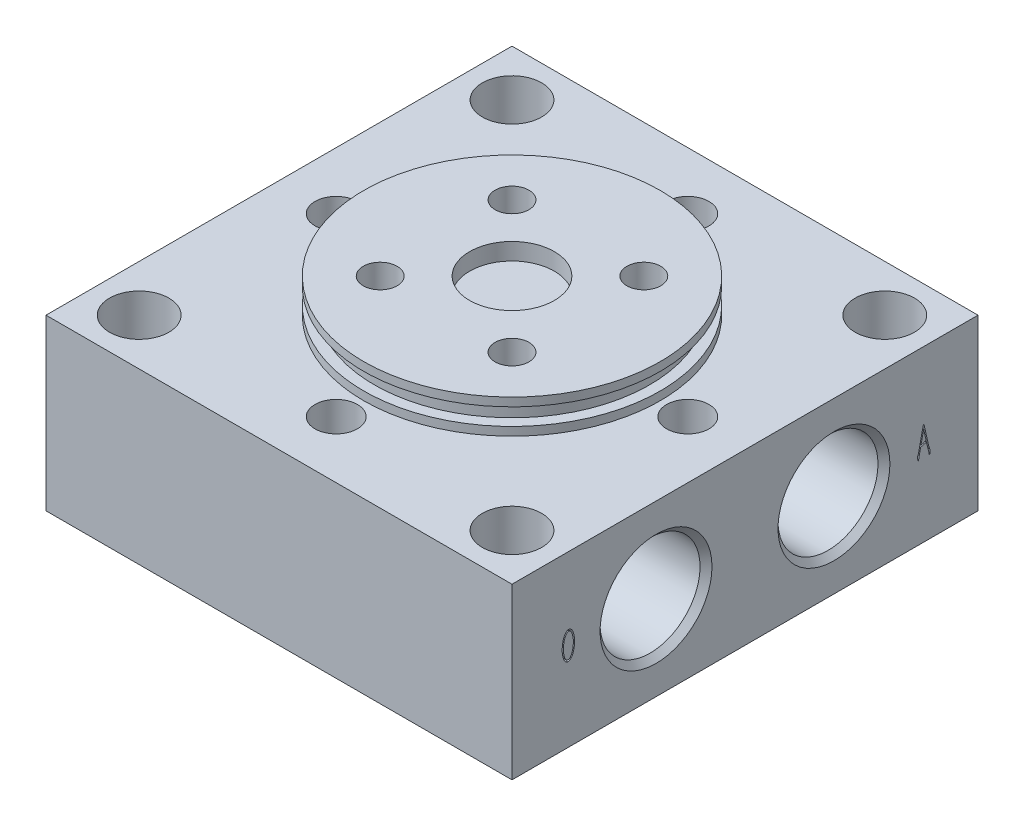
from build123d import *

# Parameters (mm, degrees)
SKETCH1_W               = 55
SKETCH1_H               = 55
BOSS_EXTRUDE1_DEPTH     = 10
SKETCH2_R               = 17.5
BOSS_EXTRUDE2_DEPTH     = 4
SKETCH3_R               = 5
CUT_EXTRUDE1_DEPTH      = 2
SKETCH4_W               = 1.25
SKETCH4_H               = 2
SKETCH9_R               = 3.5
CUT_EXTRUDE2_DEPTH      = 46.700109409
MIRROR4_COPY_1_SKETCH_R = 3.5
MIRROR4_COPY_1_DEPTH    = 46.700109409
CHAMFER1_SIZE           = 1
HOLE1_D                 = 5
HOLE1_DEPTH             = 100
HOLE1_CBORE_D           = 8.5
HOLE1_CBORE_DEPTH       = 3
CIRPATTERN1_COUNT       = 4
CHAMFER2_SIZE           = 1
CUT_EXTRUDE3_REACH      = 47.7
CUT_EXTRUDE3_END_RADIUS = 5.9
SKETCH12_R              = 2
CIRPATTERN2_COUNT       = 4
CUT_EXTRUDE4_DEPTH      = 1
CUT_EXTRUDE6_DEPTH      = 1
CUT_EXTRUDE7_DEPTH      = 1


with BuildPart() as part:
    # Sketch1 → Boss-Extrude1 (new, symmetric)
    with BuildSketch(Plane(origin=(0, 0, 0), x_dir=(1, 0, 0), z_dir=(0, 1, 0))):
        Rectangle(SKETCH1_W, SKETCH1_H)
    extrude(amount=BOSS_EXTRUDE1_DEPTH, both=True)

    # Sketch2 → Boss-Extrude2 (add)
    with BuildSketch(Plane(origin=(0, 10, 0), x_dir=(1, 0, 0), z_dir=(0, 1, 0))):
        with Locations(Location((0, 0, 0), (0, 0, 270))):
            Circle(SKETCH2_R)
    extrude(amount=BOSS_EXTRUDE2_DEPTH)

    # Sketch3 → Cut-Extrude1 (cut)
    with BuildSketch(Plane(origin=(0, 14, 0), x_dir=(1, 0, 0), z_dir=(0, 1, 0))):
        with Locations(Location((0, 0, 0), (0, 0, 270))):
            Circle(SKETCH3_R)
    extrude(amount=-CUT_EXTRUDE1_DEPTH, mode=Mode.SUBTRACT)

    # Sketch4 → Cut-Revolve1 (revolve, cut)
    with BuildSketch(Plane.XY, mode=Mode.PRIVATE) as cut_revolve1_sk:
        with Locations((-16.875, 12)):
            Rectangle(SKETCH4_W, SKETCH4_H)
    revolve(cut_revolve1_sk.sketch.rotate(Axis((0, 0, 0), (0, 1, 0)), 270), axis=Axis((0, 0, 0), (0, 1, 0)), mode=Mode.SUBTRACT)

    # Sketch6 → G1/4 Tapped Hole1 (revolve, cut)
    with BuildSketch(Plane(origin=(-27.5, 0, -10.5), x_dir=(0, 0, 1), z_dir=(0, 1, 0))):
        Polygon((0, 0), (0, 25.545077652), (5.9, 22), (5.9, 0.7035), (6.6035, 0), align=None)
    g1_4_tapped_hole1 = revolve(axis=Axis((-33.85, 0, -10.5), (1, 0, 0)), mode=Mode.SUBTRACT)

    # Mirror1: G1/4 Tapped Hole1 across plane
    add(g1_4_tapped_hole1.mirror(Plane.XY), mode=Mode.SUBTRACT)

    # Mirror2: G1/4 Tapped Hole1 across plane
    add(g1_4_tapped_hole1.mirror(Plane(origin=(0, 0, 0), x_dir=(0, 0, 1), z_dir=(1, 0, 0))), mode=Mode.SUBTRACT)

    # Mirror2 copy 1 sketch → Mirror2 copy 1 (revolve, cut)
    with BuildSketch(Plane(origin=(27.5, 0, 10.5), x_dir=(0, 0, -1), z_dir=(0, 1, 0))):
        Polygon((0, 0), (0, 25.545077652), (5.9, 22), (5.9, 0.7035), (6.6035, 0), align=None)
    revolve(axis=Axis((33.85, 0, 10.5), (-1, 0, 0)), mode=Mode.SUBTRACT)

    # Sketch9 → Cut-Extrude2 (cut, through all)
    with BuildSketch(Plane.XZ.offset(10)):
        with Locations(Location((22, 22, 0), (0, 0, 270))):
            Circle(SKETCH9_R)
    cut_extrude2 = extrude(amount=-CUT_EXTRUDE2_DEPTH, mode=Mode.SUBTRACT)

    # Mirror3: Cut-Extrude2 across plane
    add(cut_extrude2.mirror(Plane(origin=(0, 0, 0), x_dir=(0, 0, 1), z_dir=(1, 0, 0))), mode=Mode.SUBTRACT)

    # Mirror4: Cut-Extrude2 across plane
    add(cut_extrude2.mirror(Plane.XY), mode=Mode.SUBTRACT)

    # Mirror4 copy 1 sketch → Mirror4 copy 1 (cut, through all)
    with BuildSketch(Plane(origin=(0, -10, 0), x_dir=(-1, 0, 0), z_dir=(0, -1, 0))):
        with Locations(Location((22, 22, 0), (0, 0, 270))):
            Circle(MIRROR4_COPY_1_SKETCH_R)
    extrude(amount=-MIRROR4_COPY_1_DEPTH, mode=Mode.SUBTRACT)

    # Chamfer1
    chamfer1_edges = [part.edges().sort_by_distance(p)[0] for p in [
        (22, -10, 25.5),
        (-22, -10, 25.5),
        (-22, -10, -25.5),
        (22, -10, -25.5),
    ]]
    chamfer(chamfer1_edges, length=CHAMFER1_SIZE)

    # Hole1
    with Locations(Plane(origin=(0, -10, 0), x_dir=(-1, 0, 0), z_dir=(0, -1, 0))):
        with Locations((0, 20.75)):
            hole1 = CounterBoreHole(HOLE1_D / 2, HOLE1_CBORE_D / 2, HOLE1_CBORE_DEPTH, depth=HOLE1_DEPTH)

    # CirPattern1: Hole1 ×4 about axis
    cirpattern1_axis = Axis((0, 0, 0), (0, 1, 0))
    for i in range(1, CIRPATTERN1_COUNT):
        add(hole1.rotate(cirpattern1_axis, i * 360 / CIRPATTERN1_COUNT), mode=Mode.SUBTRACT)

    # Chamfer2
    chamfer2_edges = [part.edges().sort_by_distance(p)[0] for p in [
        (4.25, -10, -20.75),
        (20.75, -10, 4.25),
        (-4.25, -10, 20.75),
        (-20.75, -10, -4.25),
    ]]
    chamfer(chamfer2_edges, length=CHAMFER2_SIZE)

    # Cut-Extrude3: up to this cylinder (the profile starts outside it)
    cut_extrude3_end = Plane(origin=(-7.778175, 0, -10.5), z_dir=(-1, 0, 0)) * Cylinder(CUT_EXTRUDE3_END_RADIUS, 108.2, mode=Mode.PRIVATE)
    # Sketch12 → Cut-Extrude3 (cut, up to the surface)
    with BuildSketch(Plane(origin=(0, 14, 0), x_dir=(1, 0, 0), z_dir=(0, 1, 0)), mode=Mode.PRIVATE) as cut_extrude3_sk1:
        with Locations(Location((-7.778174593, 7.778174593, 0), (0, 0, 270))):
            Circle(SKETCH12_R)
    cut_extrude3_tool1 = extrude(cut_extrude3_sk1.sketch, amount=-CUT_EXTRUDE3_REACH, mode=Mode.PRIVATE) - cut_extrude3_end
    cut_extrude3 = cut_extrude3_tool1.solids().sort_by_distance((-7.778175, 14, -7.778175))[0]
    add(cut_extrude3, mode=Mode.SUBTRACT)

    # CirPattern2: Cut-Extrude3 ×4 about axis
    cirpattern2_axis = Axis((0, 0, 0), (0, 1, 0))
    for i in range(1, CIRPATTERN2_COUNT):
        add(cut_extrude3.rotate(cirpattern2_axis, i * 360 / CIRPATTERN2_COUNT), mode=Mode.SUBTRACT)

    # Sketch13 → Cut-Extrude4 (cut)
    with BuildSketch(Plane(origin=(27.5, 0, 0), x_dir=(0, 0, -1), z_dir=(1, 0, 0))):
        with BuildLine():
            Line((21.41827741, 0.056894821), (20.733640717, -0.108670916))
            Line((20.733640717, -0.108670916), (20.572549731, -0.85893727))
            Line((20.572549731, -0.85893727), (20.496478987, -1.241528363))
            Line((20.496478987, -1.241528363), (20.466647323, -1.362346603))
            add(Edge.make_bspline(
                [(20.466647323, -1.362346603), (20.463479594, -1.370904686), (20.458137517, -1.385337094), (20.448085785, -1.402316971), (20.437055284, -1.410755091), (20.424739604, -1.412533881), (20.415500199, -1.401854686), (20.410006027, -1.388320722), (20.408361513, -1.368459439), (20.40379183, -1.342600787), (20.400934079, -1.305609162), (20.397654946, -1.277557618), (20.395797121, -1.261664736)],
                knots=[0, 0, 0, 0, 1.226577759, 2.068508672, 2.595953142, 3.064162245, 3.560072257, 4.322224954, 5.029865969, 6.20926766, 7.852322798, 10, 10, 10, 10], degree=3))
            Line((20.395797121, -1.261664736), (20.371185998, -1.050605712))
            add(Edge.make_bspline(
                [(20.371185998, -1.050605712), (20.369595159, -1.033213536), (20.366757091, -1.002185763), (20.364263432, -0.961134647), (20.364101522, -0.931516715), (20.365536736, -0.906738529), (20.37287408, -0.883306403), (20.381590798, -0.867247825), (20.38610183, -0.85893727)],
                knots=[0, 0, 0, 0, 1.603576797, 2.86079302, 3.773774944, 4.323462854, 5.1323669, 6, 6, 6, 6], degree=3))
            Line((20.38610183, -0.85893727), (20.411458744, -0.813443982))
            add(Edge.make_bspline(
                [(20.411458744, -0.813443982), (20.416889513, -0.801595135), (20.429859356, -0.773297545), (20.446281631, -0.721203273), (20.463777805, -0.653375719), (20.481407717, -0.575307408), (20.498689018, -0.499704987), (20.512494693, -0.438103226), (20.523090834, -0.397241397), (20.529982216, -0.377138015), (20.532276984, -0.370443769)],
                knots=[0, 0, 0, 0, 0.679694972, 1.623257572, 2.844174753, 4.335796169, 5.799225578, 6.891200865, 7.630779852, 8, 8, 8, 8], degree=3))
            Line((20.532276984, -0.370443769), (21.050602149, 2.030259406))
            Line((21.050602149, 2.030259406), (21.12070656, 2.030259406))
            Line((21.12070656, 2.030259406), (21.609200061, -0.128807289))
            Line((21.609200061, -0.128807289), (21.669609181, -0.380884851))
            add(Edge.make_bspline(
                [(21.669609181, -0.380884851), (21.675668779, -0.4092612), (21.68653881, -0.460164213), (21.703079907, -0.52776564), (21.716645868, -0.578389221), (21.726184983, -0.606146467), (21.730018301, -0.61730079)],
                knots=[0, 0, 0, 0, 1.425899692, 2.557855139, 3.420470246, 4, 4, 4, 4], degree=3))
            Line((21.730018301, -0.61730079), (21.765070506, -0.712762115))
            add(Edge.make_bspline(
                [(21.765070506, -0.712762115), (21.769105272, -0.726745828), (21.77645646, -0.752223612), (21.789013801, -0.785943136), (21.80135485, -0.811979223), (21.817068063, -0.833907011), (21.833006758, -0.850364641), (21.844008493, -0.867431963), (21.845398376, -0.883364804), (21.84347131, -0.897971275), (21.841413369, -0.916574349), (21.840412026, -0.939998551), (21.837753743, -0.972271763), (21.836579468, -0.996654459), (21.835920709, -1.010332965)],
                knots=[0, 0, 0, 0, 1.645080438, 2.997272953, 4.065812928, 4.892545225, 6.029861332, 6.67147811, 7.124734071, 7.80170629, 8.338742145, 9.240009017, 10.451666043, 12, 12, 12, 12], degree=3))
            Line((21.835920709, -1.010332965), (21.815784336, -1.236307822))
            Line((21.815784336, -1.236307822), (21.805343253, -1.322073856))
            add(Edge.make_bspline(
                [(21.805343253, -1.322073856), (21.804846829, -1.331800262), (21.803964414, -1.349089378), (21.799710387, -1.371359831), (21.796925261, -1.387525447), (21.791057653, -1.399220748), (21.779909712, -1.405003708), (21.766089397, -1.400970109), (21.755467273, -1.386991211), (21.752111389, -1.374721336), (21.750154674, -1.367567144)],
                knots=[0, 0, 0, 0, 1.663187075, 2.956388731, 3.874273883, 4.464983498, 5.130530035, 5.83179128, 6.735783313, 8, 8, 8, 8], degree=3))
            Line((21.750154674, -1.367567144), (21.715102469, -1.166203411))
            Line((21.715102469, -1.166203411), (21.41827741, 0.056894821))
        make_face()
        with BuildLine():
            Line((21.407836328, 0.132965564), (21.085654355, 1.546986446))
            Line((21.085654355, 1.546986446), (20.75825184, 0.067335903))
            add(Edge.make_bspline(
                [(20.75825184, 0.067335903), (20.786653818, 0.071713699), (20.835687119, 0.079271544), (20.904028724, 0.094281317), (20.968709563, 0.112048218), (21.026146573, 0.127940621), (21.073590406, 0.14406318), (21.104589464, 0.154731291), (21.128139648, 0.165754404), (21.140665789, 0.174111761), (21.146063475, 0.177713061)],
                knots=[0, 0, 0, 0, 1.70172219, 2.937860729, 4.141475294, 5.674569601, 6.46612829, 7.108957565, 7.616037637, 8, 8, 8, 8], degree=3))
            Line((21.146063475, 0.177713061), (21.272102256, 0.263479095))
            Line((21.272102256, 0.263479095), (21.407836328, 0.132965564))
        make_face(mode=Mode.SUBTRACT)
    extrude(amount=-CUT_EXTRUDE4_DEPTH, mode=Mode.SUBTRACT)

    # Sketch14 → Cut-Extrude6 (cut)
    with BuildSketch(Plane(origin=(27.5, 0, 0), x_dir=(0, 0, -1), z_dir=(1, 0, 0))):
        with BuildLine():
            add(Edge.make_bspline(
                [(-21.573757582, 0.463669295), (-21.570691446, 0.511932871), (-21.564373449, 0.611383491), (-21.546495118, 0.764033475), (-21.523391202, 0.924733609), (-21.494531327, 1.089931426), (-21.45842848, 1.253615372), (-21.409140298, 1.406968714), (-21.350380038, 1.548232182), (-21.280957443, 1.673587805), (-21.208198436, 1.781766032), (-21.137917897, 1.870157478), (-21.071763548, 1.938118373), (-21.006582548, 1.983823464), (-20.944517431, 2.012043895), (-20.887579323, 2.031645432), (-20.834254477, 2.044425119), (-20.799687025, 2.044138334), (-20.783218481, 2.044001705)],
                knots=[0, 0, 0, 0, 1.217793816, 2.509352989, 3.869389901, 5.306369188, 6.732518591, 8.086865491, 9.357865112, 10.57959578, 11.689225504, 12.637700741, 13.421327601, 14.069152645, 14.629329011, 15.132240194, 15.586583926, 16, 16, 16, 16], degree=3))
            add(Edge.make_bspline(
                [(-20.783218481, 2.044001705), (-20.767426973, 2.041261552), (-20.733849942, 2.035435245), (-20.682789884, 2.015383688), (-20.627615703, 1.987897956), (-20.569705453, 1.950672135), (-20.51151679, 1.90327457), (-20.456490892, 1.843520338), (-20.406791008, 1.771014125), (-20.345589446, 1.658264953), (-20.278997371, 1.503374055), (-20.226466165, 1.338747987), (-20.19239833, 1.199951602), (-20.16889652, 1.089116308), (-20.149948201, 0.972064152), (-20.128312505, 0.80900423), (-20.108857675, 0.601811935), (-20.111955861, 0.435372211), (-20.11349762, 0.352546346)],
                knots=[0, 0, 0, 0, 0.394985608, 0.839846589, 1.347857167, 1.916750551, 2.536277094, 3.196746505, 3.915575437, 4.701623328, 6.36253532, 8.071356979, 8.963406565, 9.891884595, 10.869033514, 11.891140732, 13.955296867, 16, 16, 16, 16], degree=3))
            add(Edge.make_bspline(
                [(-20.11349762, 0.352546346), (-20.114789645, 0.321461233), (-20.117469781, 0.256979241), (-20.125601646, 0.157428876), (-20.139029229, 0.051884429), (-20.159125682, -0.097503151), (-20.196773191, -0.288653981), (-20.248813642, -0.478020533), (-20.299959181, -0.626162428), (-20.343875525, -0.731714709), (-20.392424734, -0.831888465), (-20.446108546, -0.924275466), (-20.50188653, -1.007422099), (-20.561638755, -1.076348685), (-20.622032408, -1.131723757), (-20.684965724, -1.17077827), (-20.74573499, -1.197352301), (-20.802093274, -1.215837832), (-20.854774052, -1.224903531), (-20.888103078, -1.223826305), (-20.904036721, -1.223311315)],
                knots=[0, 0, 0, 0, 0.881282943, 1.828105941, 2.82824081, 3.894865892, 6.097710261, 8.340987808, 9.452332789, 10.535200188, 11.577677107, 12.603151353, 13.560288859, 14.408919748, 15.182050945, 15.871786862, 16.496001568, 17.057257397, 17.549302039, 18, 18, 18, 18], degree=3))
            add(Edge.make_bspline(
                [(-20.904036721, -1.223311315), (-20.920550298, -1.221349209), (-20.955215733, -1.217230342), (-21.008123304, -1.199662765), (-21.064025867, -1.173173265), (-21.123094658, -1.137571684), (-21.182895081, -1.089677604), (-21.238402903, -1.02552304), (-21.292412395, -0.948198037), (-21.341946304, -0.856675456), (-21.388278542, -0.754904909), (-21.429707213, -0.64507945), (-21.467077085, -0.529109163), (-21.499540849, -0.408405105), (-21.525554664, -0.285756755), (-21.547809745, -0.16551661), (-21.562311551, -0.048680046), (-21.572466566, 0.063757537), (-21.576060976, 0.171547051), (-21.578741939, 0.273970972), (-21.578200055, 0.370740853), (-21.575207138, 0.43334721), (-21.573757582, 0.463669295)],
                knots=[0, 0, 0, 0, 0.510534934, 1.071719088, 1.704710998, 2.411693894, 3.189282936, 4.05053371, 5.011670478, 6.086573801, 7.246791516, 8.449877322, 9.695482973, 10.994127406, 12.29322218, 13.551907867, 14.754774865, 15.913908135, 17.0238299, 18.071869134, 19.066149983, 20, 20, 20, 20], degree=3))
        make_face()
        with BuildLine():
            add(Edge.make_bspline(
                [(-21.427582427, 0.453228212), (-21.428993902, 0.42837503), (-21.431970413, 0.375964764), (-21.433120165, 0.293132799), (-21.432450524, 0.202116471), (-21.427658159, 0.068578079), (-21.41028584, -0.107700957), (-21.379671203, -0.28600609), (-21.345210741, -0.427946487), (-21.315480687, -0.529686707), (-21.282797293, -0.626028097), (-21.246040906, -0.714982753), (-21.206989611, -0.795194849), (-21.16389052, -0.86269606), (-21.120795203, -0.919498218), (-21.07284554, -0.96095983), (-21.026449208, -0.993065397), (-20.981582585, -1.014859935), (-20.939913724, -1.031579991), (-20.912122244, -1.035152811), (-20.89881618, -1.036863414)],
                knots=[0, 0, 0, 0, 0.796536737, 1.679732718, 2.650327695, 3.709147218, 5.954918549, 8.313069364, 9.492003862, 10.627402775, 11.704181224, 12.745734999, 13.706334556, 14.553839847, 15.30675304, 15.97732542, 16.573080319, 17.10674674, 17.572326302, 18, 18, 18, 18], degree=3))
            add(Edge.make_bspline(
                [(-20.89881618, -1.036863414), (-20.885116088, -1.03766974), (-20.856757889, -1.039338778), (-20.813193016, -1.030783983), (-20.767605376, -1.015733546), (-20.720395542, -0.991454463), (-20.671471858, -0.956768819), (-20.624678335, -0.906675445), (-20.577997255, -0.843572885), (-20.532200589, -0.768401348), (-20.48815732, -0.685034131), (-20.449030213, -0.595717941), (-20.412653191, -0.503480042), (-20.372741813, -0.374175287), (-20.328733755, -0.207848896), (-20.294142862, -0.00469703), (-20.270054835, 0.193469365), (-20.257219824, 0.354343807), (-20.255310839, 0.482324845), (-20.257833517, 0.585540018), (-20.263512534, 0.697752569), (-20.2708083, 0.775432835), (-20.274588607, 0.815682932)],
                knots=[0, 0, 0, 0, 0.389303871, 0.805830913, 1.253424913, 1.753499798, 2.311288848, 2.951911425, 3.695005091, 4.54345845, 5.455166886, 6.377091015, 7.318103512, 8.276048787, 10.227707478, 12.21152619, 14.136557685, 15.91040834, 16.802233067, 17.779101204, 18.849239395, 20, 20, 20, 20], degree=3))
            add(Edge.make_bspline(
                [(-20.274588607, 0.815682932), (-20.278749151, 0.85227031), (-20.286835512, 0.923380897), (-20.303712465, 1.025706179), (-20.321026259, 1.121196747), (-20.349319536, 1.238195031), (-20.390241956, 1.379672869), (-20.442858772, 1.515193259), (-20.490824524, 1.617126524), (-20.529489874, 1.683357874), (-20.573518157, 1.737161993), (-20.619504542, 1.779802429), (-20.666198859, 1.811647703), (-20.71008361, 1.836185545), (-20.752407674, 1.852061459), (-20.780378775, 1.855785577), (-20.793659563, 1.857553804)],
                knots=[0, 0, 0, 0, 1.251575308, 2.432539829, 3.524812851, 4.549720602, 6.523204923, 8.527303315, 9.483611249, 10.351763581, 11.126540771, 11.838283349, 12.475927762, 13.043152764, 13.545685196, 14, 14, 14, 14], degree=3))
            add(Edge.make_bspline(
                [(-20.793659563, 1.857553804), (-20.8066188, 1.85661231), (-20.834081233, 1.854617153), (-20.876887901, 1.845024545), (-20.921372027, 1.825740368), (-20.971141922, 1.802471809), (-21.023638907, 1.76325926), (-21.076807726, 1.704111951), (-21.132758519, 1.62563128), (-21.192555488, 1.530306852), (-21.249824351, 1.418473241), (-21.296642695, 1.290920724), (-21.33756029, 1.151604218), (-21.365700214, 1.002386979), (-21.389120424, 0.853049539), (-21.406566885, 0.710439818), (-21.421041536, 0.578506064), (-21.425465251, 0.49377853), (-21.427582427, 0.453228212)],
                knots=[0, 0, 0, 0, 0.37757334, 0.800130614, 1.267198275, 1.784369715, 2.394414205, 3.156344445, 4.08734282, 5.194407036, 6.425938495, 7.73207238, 9.1388751, 10.642807986, 12.142427514, 13.533772035, 14.819671431, 16, 16, 16, 16], degree=3))
        make_face(mode=Mode.SUBTRACT)
    extrude(amount=-CUT_EXTRUDE6_DEPTH, mode=Mode.SUBTRACT)

    # Sketch15 → Cut-Extrude7 (cut)
    # profile 1 of 2: a face of its own
    with BuildSketch(Plane.ZY.offset(27.5)):
        with BuildLine():
            add(Edge.make_bspline(
                [(-22.716854148, 1.943319838), (-22.678283366, 1.949836343), (-22.604277282, 1.962339617), (-22.496871122, 1.983743416), (-22.393200184, 2.001804845), (-22.324140124, 2.006563605), (-22.289515559, 2.008949499)],
                knots=[0, 0, 0, 0, 1.084781132, 2.081378719, 3.038062992, 4, 4, 4, 4], degree=3))
            add(Edge.make_bspline(
                [(-22.289515559, 2.008949499), (-22.269612591, 2.009379341), (-22.231712494, 2.010197864), (-22.178043644, 2.004711516), (-22.130099478, 1.99577851), (-22.087718008, 1.979371435), (-22.048808231, 1.957200452), (-22.011532761, 1.927956184), (-21.975273294, 1.891371922), (-21.939913694, 1.846869118), (-21.906856359, 1.79404757), (-21.879514156, 1.73085753), (-21.856212079, 1.658519117), (-21.835491489, 1.550364095), (-21.815180708, 1.414048318), (-21.808170117, 1.279654783), (-21.80790067, 1.179100032), (-21.810863807, 1.11041887), (-21.816441375, 1.046873921), (-21.823154397, 1.006573268), (-21.826378972, 0.987215001)],
                knots=[0, 0, 0, 0, 0.834042403, 1.588219797, 2.258865872, 2.872645434, 3.484296274, 4.130763207, 4.85321558, 5.639635085, 6.510463327, 7.457868132, 8.519533185, 9.691141985, 12.070813463, 14.294972691, 15.327100164, 16.287155067, 17.177241371, 18, 18, 18, 18], degree=3))
            add(Edge.make_bspline(
                [(-21.826378972, 0.987215001), (-21.830486178, 0.964508438), (-21.83849221, 0.92024733), (-21.856297246, 0.85702977), (-21.875017714, 0.797567908), (-21.89836069, 0.74383886), (-21.922884912, 0.694379821), (-21.950358068, 0.650866263), (-21.97950663, 0.611880349), (-22.0214278, 0.569497691), (-22.077733739, 0.526608018), (-22.151540319, 0.493581811), (-22.226174894, 0.477633394), (-22.275286261, 0.474762931), (-22.299210849, 0.473364586)],
                knots=[0, 0, 0, 0, 1.080384674, 2.105956013, 3.074594822, 3.998289199, 4.84730105, 5.658400013, 6.406150959, 7.122683501, 8.445750941, 9.696890862, 10.878041055, 12, 12, 12, 12], degree=3))
            Line((-22.299210849, 0.473364586), (-22.495354041, 0.463669295))
            Line((-22.495354041, 0.463669295), (-22.757126895, 0.427871298))
            Line((-22.757126895, 0.427871298), (-22.762347436, -0.921265715))
            add(Edge.make_bspline(
                [(-22.762347436, -0.921265715), (-22.762913705, -0.951104576), (-22.76393324, -1.004827776), (-22.767620667, -1.076370903), (-22.768976187, -1.130408058), (-22.773464208, -1.180316008), (-22.778647003, -1.235510532), (-22.785967882, -1.288051036), (-22.791634518, -1.329651282), (-22.797623402, -1.34918199), (-22.802940506, -1.365782803), (-22.810361882, -1.364670505), (-22.813061265, -1.364265928)],
                knots=[0, 0, 0, 0, 1.96874048, 3.54460707, 4.726507013, 5.532831549, 6.851459339, 8.37313705, 9.071482733, 9.549088405, 9.835989539, 10, 10, 10, 10], degree=3))
            add(Edge.make_bspline(
                [(-22.813061265, -1.364265928), (-22.814050257, -1.363515116), (-22.818283382, -1.360301457), (-22.828625097, -1.353594461), (-22.839143721, -1.334273174), (-22.844737765, -1.318094511), (-22.84811347, -1.308331558)],
                knots=[0, 0, 0, 0, 0.220639879, 0.944392497, 2.156105254, 4, 4, 4, 4], degree=3))
            Line((-22.84811347, -1.308331558), (-22.873470385, -1.243447688))
            Line((-22.873470385, -1.243447688), (-22.933879505, -1.062220328))
            add(Edge.make_bspline(
                [(-22.933879505, -1.062220328), (-22.939513362, -1.044804713), (-22.94933033, -1.014458094), (-22.962969508, -0.975502701), (-22.969638556, -0.949202442), (-22.973423325, -0.928583645), (-22.964353832, -0.908163009), (-22.952948275, -0.880410812), (-22.937203358, -0.844065308), (-22.925904097, -0.799188809), (-22.915119575, -0.751163059), (-22.905346196, -0.700553929), (-22.899308598, -0.644979539), (-22.897724549, -0.591886551), (-22.898520003, -0.539408434), (-22.895984535, -0.48698194), (-22.896276463, -0.423306829), (-22.894540329, -0.377082761), (-22.893606758, -0.352226721)],
                knots=[0, 0, 0, 0, 1.21093634, 2.110050319, 2.719907809, 3.017552618, 3.464624392, 4.142243825, 5.027278712, 6.067997939, 7.196380019, 8.282686609, 9.473265847, 10.887508473, 11.791416163, 12.942313598, 14.355792079, 16, 16, 16, 16], degree=3))
            Line((-22.893606758, -0.352226721), (-22.883165676, 1.721819732))
            add(Edge.make_bspline(
                [(-22.883165676, 1.721819732), (-22.89393359, 1.743438266), (-22.913721033, 1.783165134), (-22.946094396, 1.833417418), (-22.971246853, 1.87169286), (-22.984027246, 1.9020465), (-22.987699799, 1.92482587), (-22.988644728, 1.937597694), (-22.989068084, 1.943319838)],
                knots=[0, 0, 0, 0, 1.750659444, 3.217064329, 4.333728491, 5.070582308, 5.583594197, 6, 6, 6, 6], degree=3))
            add(Edge.make_bspline(
                [(-22.989068084, 1.943319838), (-22.988395861, 1.946273967), (-22.986846978, 1.953080635), (-22.974941937, 1.958979274), (-22.95853723, 1.959110016), (-22.94582175, 1.958559169), (-22.938354254, 1.95823567)],
                knots=[0, 0, 0, 0, 0.599620471, 1.381597738, 2.462275397, 4, 4, 4, 4], degree=3))
            Line((-22.938354254, 1.95823567), (-22.888386217, 1.948540379))
            Line((-22.888386217, 1.948540379), (-22.716854148, 1.943319838))
        make_face()
        with BuildLine():
            Line((-22.757126895, 0.604623908), (-22.420029089, 0.639676113))
            add(Edge.make_bspline(
                [(-22.420029089, 0.639676113), (-22.389659167, 0.64277566), (-22.325531551, 0.649320508), (-22.24450315, 0.664153492), (-22.17912965, 0.68387545), (-22.132739522, 0.703769588), (-22.092221091, 0.730318638), (-22.056122995, 0.761985542), (-22.026096533, 0.801171941), (-22.000039453, 0.846962008), (-21.98233073, 0.901671976), (-21.963625288, 0.984329257), (-21.950018717, 1.095916352), (-21.948147345, 1.187053907), (-21.947197212, 1.233326231)],
                knots=[0, 0, 0, 0, 1.242290402, 2.623158502, 3.343124827, 4.017967388, 4.668958523, 5.306607609, 5.962297971, 6.668776287, 7.439809609, 8.291324773, 10.117032856, 12, 12, 12, 12], degree=3))
            add(Edge.make_bspline(
                [(-21.947197212, 1.233326231), (-21.949190047, 1.262682698), (-21.953081569, 1.320008764), (-21.962820803, 1.403109396), (-21.975159968, 1.481396301), (-21.991809279, 1.553409649), (-22.008933129, 1.618648883), (-22.031858427, 1.673582275), (-22.055811912, 1.719079423), (-22.084068796, 1.755260629), (-22.117983756, 1.781769735), (-22.155541079, 1.804450295), (-22.200583979, 1.818616365), (-22.232522474, 1.824593178), (-22.249242812, 1.827722139)],
                knots=[0, 0, 0, 0, 1.450841259, 2.833141438, 4.12506739, 5.356415584, 6.477956507, 7.445537896, 8.28503356, 9.008768821, 9.688489171, 10.397114349, 11.160862483, 12, 12, 12, 12], degree=3))
            add(Edge.make_bspline(
                [(-22.249242812, 1.827722139), (-22.271617187, 1.828905835), (-22.317132287, 1.83131377), (-22.387413565, 1.826636657), (-22.460791645, 1.818330974), (-22.510339715, 1.807760111), (-22.535626788, 1.802365225)],
                knots=[0, 0, 0, 0, 0.931107193, 1.894105981, 2.925247858, 4, 4, 4, 4], degree=3))
            Line((-22.535626788, 1.802365225), (-22.742211062, 1.756871937))
            Line((-22.742211062, 1.756871937), (-22.757126895, 0.604623908))
        make_face(mode=Mode.SUBTRACT)
    # profile 2 of 2: a face of its own
    with BuildSketch(Plane.ZY.offset(27.5)):
        with BuildLine():
            add(Edge.make_bspline(
                [(21.693628067, 1.691988067), (21.68144982, 1.701426351), (21.659363699, 1.718543354), (21.626261092, 1.744287943), (21.595203373, 1.778112565), (21.566001926, 1.809561073), (21.542963494, 1.838354352), (21.531298815, 1.857622523), (21.523402988, 1.872579283), (21.5246256, 1.887945488), (21.533040377, 1.899696569), (21.541193258, 1.915088033), (21.563602484, 1.919215799), (21.588357215, 1.909906461), (21.614687366, 1.902080584), (21.635412693, 1.895266882), (21.653617141, 1.894705762), (21.675240608, 1.894612962), (21.706296294, 1.896767623), (21.744122071, 1.89751905), (21.782487322, 1.900134297), (21.815655143, 1.904454798), (21.841014373, 1.906760924), (21.85451463, 1.91155979), (21.859939594, 1.913488174)],
                knots=[0, 0, 0, 0, 1.64763205, 2.988098512, 4.472525849, 6.542356651, 7.584071831, 8.395257026, 8.967619365, 9.340564694, 9.97047718, 10.50190227, 11.107820098, 12.171334353, 13.314207223, 14.055349962, 14.481319576, 15.251885957, 16.369143228, 17.804974755, 19.296756072, 20.473415709, 21.386554954, 22, 22, 22, 22], degree=3))
            Line((21.859939594, 1.913488174), (22.112017157, 1.978372043))
            add(Edge.make_bspline(
                [(22.112017157, 1.978372043), (22.119702955, 1.98044976), (22.136711154, 1.98504762), (22.165526756, 1.990525658), (22.199458045, 1.998322566), (22.237580097, 2.005832569), (22.275388858, 2.014366522), (22.309884837, 2.018912641), (22.338365704, 2.023636951), (22.355627879, 2.02379475), (22.363348927, 2.023865331)],
                knots=[0, 0, 0, 0, 0.746644526, 1.652278328, 2.750112717, 4.012480095, 5.297690843, 6.382818677, 7.276664985, 8, 8, 8, 8], degree=3))
            add(Edge.make_bspline(
                [(22.363348927, 2.023865331), (22.37982691, 2.022072977), (22.412751277, 2.018491706), (22.461110029, 2.005058118), (22.507028119, 1.982656487), (22.550925834, 1.953858233), (22.59095464, 1.917821047), (22.627459229, 1.876311777), (22.658758162, 1.828330499), (22.684805886, 1.773689163), (22.706945512, 1.71319037), (22.72584969, 1.645908965), (22.740102535, 1.571731472), (22.751667489, 1.492807566), (22.760330626, 1.413671477), (22.766178377, 1.338293148), (22.770179572, 1.268917079), (22.770935959, 1.224630002), (22.771296935, 1.203494566)],
                knots=[0, 0, 0, 0, 0.788100513, 1.574689806, 2.373814472, 3.210589555, 4.065404581, 4.929098289, 5.834801075, 6.781980012, 7.803943584, 8.897694274, 10.10426717, 11.396006919, 12.693423483, 13.892139677, 14.994050896, 16, 16, 16, 16], degree=3))
            add(Edge.make_bspline(
                [(22.771296935, 1.203494566), (22.769145225, 1.169656343), (22.764799581, 1.10131587), (22.751972016, 0.997937392), (22.732724057, 0.891869128), (22.709802435, 0.804084814), (22.688794175, 0.738272076), (22.672903369, 0.698999764), (22.658719328, 0.668878774), (22.645550138, 0.65512756), (22.640037613, 0.649371404)],
                knots=[0, 0, 0, 0, 1.41233288, 2.852380741, 4.337314802, 5.89979107, 6.630150315, 7.21096505, 7.669715816, 8, 8, 8, 8], degree=3))
            Line((22.640037613, 0.649371404), (22.534880996, 0.544214788))
            add(Edge.make_bspline(
                [(22.534880996, 0.544214788), (22.557565411, 0.528722792), (22.598608356, 0.500693102), (22.645071678, 0.461390329), (22.678319315, 0.427877598), (22.70281792, 0.394674541), (22.73083987, 0.354139497), (22.770492123, 0.288189414), (22.817818257, 0.194199685), (22.847914883, 0.088254297), (22.866218398, -0.004931345), (22.873392474, -0.084855293), (22.878294161, -0.17292535), (22.877574807, -0.234383111), (22.877199343, -0.266460686)],
                knots=[0, 0, 0, 0, 1.070182896, 1.936283469, 2.368030692, 2.906882123, 3.541225939, 4.289096852, 5.905680189, 7.625612947, 8.562596306, 9.604952081, 10.749916543, 12, 12, 12, 12], degree=3))
            add(Edge.make_bspline(
                [(22.877199343, -0.266460686), (22.8759769, -0.296803371), (22.873598293, -0.355843629), (22.865639768, -0.442058005), (22.852471261, -0.523298732), (22.837622633, -0.60003388), (22.817272823, -0.671322376), (22.793079988, -0.736902963), (22.763747766, -0.796750681), (22.729229762, -0.850591225), (22.690355116, -0.89946799), (22.646336534, -0.943206688), (22.597905074, -0.982730633), (22.544625307, -1.017813007), (22.487612402, -1.048444602), (22.426168859, -1.072985294), (22.361430264, -1.093488422), (22.316221662, -1.102425553), (22.293244517, -1.106967824)],
                knots=[0, 0, 0, 0, 1.291181941, 2.512358873, 3.678492505, 4.789671877, 5.833657235, 6.827132701, 7.758433233, 8.661592748, 9.541502867, 10.408556622, 11.295108621, 12.19516981, 13.117306623, 14.041863747, 15.004782726, 16, 16, 16, 16], degree=3))
            Line((22.293244517, -1.106967824), (22.000894208, -1.147240571))
            add(Edge.make_bspline(
                [(22.000894208, -1.147240571), (21.985259933, -1.149926812), (21.955793543, -1.154989651), (21.914273998, -1.159075843), (21.878961301, -1.165532537), (21.841216877, -1.168088833), (21.801252065, -1.175440191), (21.765194961, -1.19609055), (21.746205554, -1.218513359), (21.73325, -1.225672875), (21.729426064, -1.227786064)],
                knots=[0, 0, 0, 0, 1.312917143, 2.474494646, 3.452532002, 4.279929402, 5.608244096, 6.780169529, 7.639957153, 8, 8, 8, 8], degree=3))
            add(Edge.make_bspline(
                [(21.729426064, -1.227786064), (21.725579874, -1.228212546), (21.715830621, -1.229293584), (21.704856101, -1.218831948), (21.692882261, -1.207464523), (21.677035192, -1.19538196), (21.657258634, -1.178549673), (21.623974872, -1.154294575), (21.585240763, -1.120690776), (21.548630463, -1.07854583), (21.525239678, -1.041994266), (21.512153955, -1.01271209), (21.5096927, -0.994566793), (21.508460636, -0.979570213), (21.527146568, -0.974602453), (21.539483868, -0.972628275), (21.548198704, -0.971233752)],
                knots=[0, 0, 0, 0, 0.408406666, 1.035221836, 1.516918604, 2.252554637, 3.200824533, 4.366195779, 6.758465887, 8.80503204, 10.444321207, 11.5313617, 12.220697094, 12.548554928, 12.974726626, 14, 14, 14, 14], degree=3))
            Line((21.548198704, -0.971233752), (21.693628067, -0.971233752))
            Line((21.693628067, -0.971233752), (21.693628067, 1.691988067))
        make_face()
        with BuildLine():
            Line((21.824887389, 0.584487535), (22.222394314, 0.629235031))
            add(Edge.make_bspline(
                [(22.222394314, 0.629235031), (22.24278608, 0.631910893), (22.281129761, 0.636942454), (22.334407914, 0.644813806), (22.379346656, 0.653353648), (22.417953864, 0.660640646), (22.452190714, 0.674426681), (22.482227851, 0.697899534), (22.510240593, 0.729356358), (22.544149641, 0.782735081), (22.581204596, 0.857170946), (22.612342376, 0.954052052), (22.632552215, 1.05619826), (22.636397595, 1.163208169), (22.635357521, 1.271351381), (22.635494888, 1.343700004), (22.635562863, 1.379501385)],
                knots=[0, 0, 0, 0, 0.873777503, 1.643008589, 2.287243073, 2.817622504, 3.309938555, 3.837999608, 4.421262104, 5.092045153, 6.518435707, 7.941185456, 9.403523715, 10.926684676, 12.47918417, 14, 14, 14, 14], degree=3))
            add(Edge.make_bspline(
                [(22.635562863, 1.379501385), (22.633893881, 1.401912033), (22.630712383, 1.444632324), (22.621167211, 1.505212865), (22.611418567, 1.559435117), (22.594769121, 1.621383565), (22.567227335, 1.689999904), (22.525214915, 1.747236107), (22.486982777, 1.783574231), (22.457658351, 1.805479922), (22.42595568, 1.819616593), (22.384313706, 1.829704739), (22.335606096, 1.834246574), (22.288731077, 1.831874967), (22.251711203, 1.825071469), (22.218555046, 1.819345849), (22.179690061, 1.810792699), (22.151556244, 1.805286726), (22.13662828, 1.802365225)],
                knots=[0, 0, 0, 0, 1.337822755, 2.550224273, 3.650783, 4.616944903, 6.368664393, 8.021145033, 8.796181901, 9.507039394, 10.189576941, 10.84675067, 12.051897664, 13.090030714, 13.630410622, 14.292569305, 15.094027531, 16, 16, 16, 16], degree=3))
            Line((22.13662828, 1.802365225), (21.824887389, 1.721819732))
            Line((21.824887389, 1.721819732), (21.824887389, 0.584487535))
        make_face(mode=Mode.SUBTRACT)
        with BuildLine():
            add(Edge.make_bspline(
                [(21.824887389, -0.971233752), (21.846506849, -0.972837252), (21.886239064, -0.975784161), (21.940218898, -0.978241849), (21.983246945, -0.978185336), (22.018419996, -0.977116749), (22.052547644, -0.971969451), (22.092248452, -0.968467683), (22.14052275, -0.960669092), (22.21465948, -0.952377993), (22.306425844, -0.93450922), (22.394658041, -0.911706451), (22.458064541, -0.883330784), (22.502195853, -0.853719083), (22.544550175, -0.815966897), (22.59516376, -0.754616455), (22.651213085, -0.674202244), (22.69675057, -0.571065983), (22.726798926, -0.46940192), (22.739788257, -0.368021233), (22.744293682, -0.268720443), (22.741901485, -0.203316191), (22.740719479, -0.170999361)],
                knots=[0, 0, 0, 0, 0.898162711, 1.650642252, 2.237699247, 2.68104558, 3.106443072, 3.666024881, 4.33166218, 5.131363942, 6.755447525, 8.202702255, 8.893980373, 9.622392647, 10.39559097, 11.23565845, 12.912443945, 14.438192962, 15.885447693, 17.289548788, 18.660741617, 20, 20, 20, 20], degree=3))
            add(Edge.make_bspline(
                [(22.740719479, -0.170999361), (22.736703827, -0.129140534), (22.728980389, -0.048632043), (22.706449312, 0.066299852), (22.671851612, 0.170535611), (22.618570928, 0.26011459), (22.553410863, 0.335263126), (22.47798766, 0.391801662), (22.400668634, 0.429548207), (22.334674959, 0.448068387), (22.277650436, 0.452471856), (22.223605071, 0.453037032), (22.156693437, 0.449536432), (22.108028328, 0.44565408), (22.081439701, 0.443532921)],
                knots=[0, 0, 0, 0, 1.438130322, 2.76600445, 4.000792246, 5.175154235, 6.308219456, 7.383388526, 8.376306419, 9.238740087, 9.708503365, 10.329505009, 11.087309779, 12, 12, 12, 12], degree=3))
            Line((22.081439701, 0.443532921), (21.824887389, 0.412955466))
            Line((21.824887389, 0.412955466), (21.824887389, -0.971233752))
        make_face(mode=Mode.SUBTRACT)
    extrude(amount=-CUT_EXTRUDE7_DEPTH, mode=Mode.SUBTRACT)


solid = part.part
